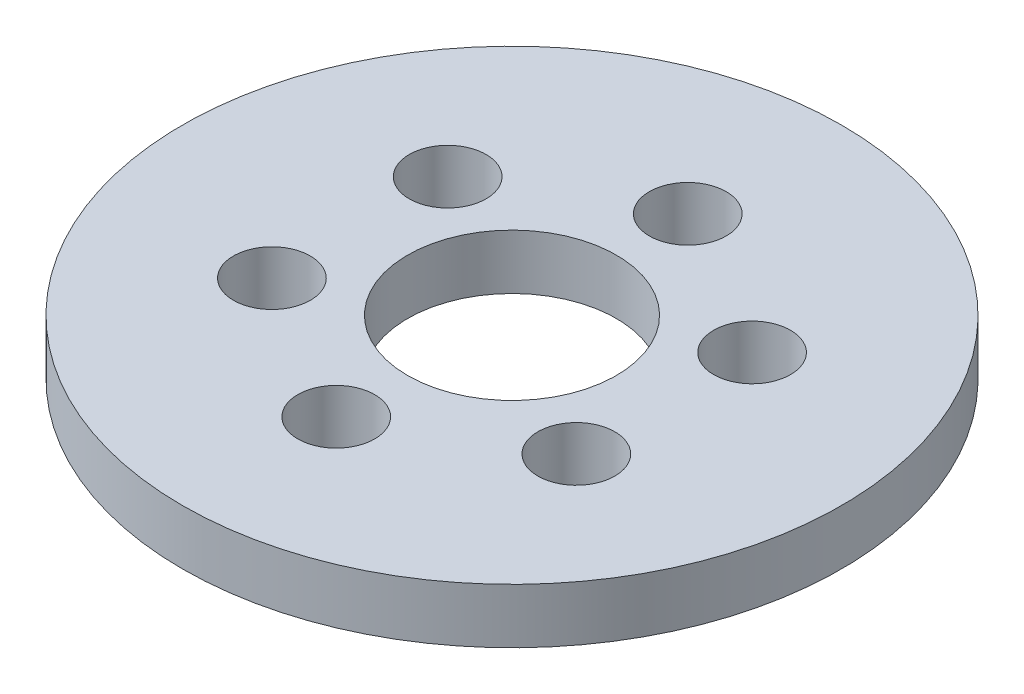
from build123d import *

# Parameters (mm, degrees)
SKETCH_1_R         = 30
SKETCH_1_R_2       = 9.5
EXTRUDE_1_DEPTH    = 5
HOLE_WIZARD_M6_1_D = 7


with BuildPart() as part:
    # 草图1 → 凸台-拉伸1 (new body)
    with BuildSketch(Plane(origin=(0, 0, 0), x_dir=(1, 0, 0), z_dir=(0, 1, 0))):
        with Locations(Location((0, 0, 0), (0, 0, 270))):
            Circle(SKETCH_1_R)
        with Locations(Location((0, 0, 0), (0, 0, 270))):
            Circle(SKETCH_1_R_2, mode=Mode.SUBTRACT)
    extrude(amount=EXTRUDE_1_DEPTH)

    # M6 间隙孔1 (through all)
    with Locations(Plane(origin=(0, 5, 0), x_dir=(1, 0, 0), z_dir=(0, 1, 0))):
        with Locations((0, 16), (13.856406461, 8), (13.856406461, -8), (0, -16), (-13.856406461, -8), (-13.856406461, 8)):
            Hole(HOLE_WIZARD_M6_1_D / 2)


solid = part.part
